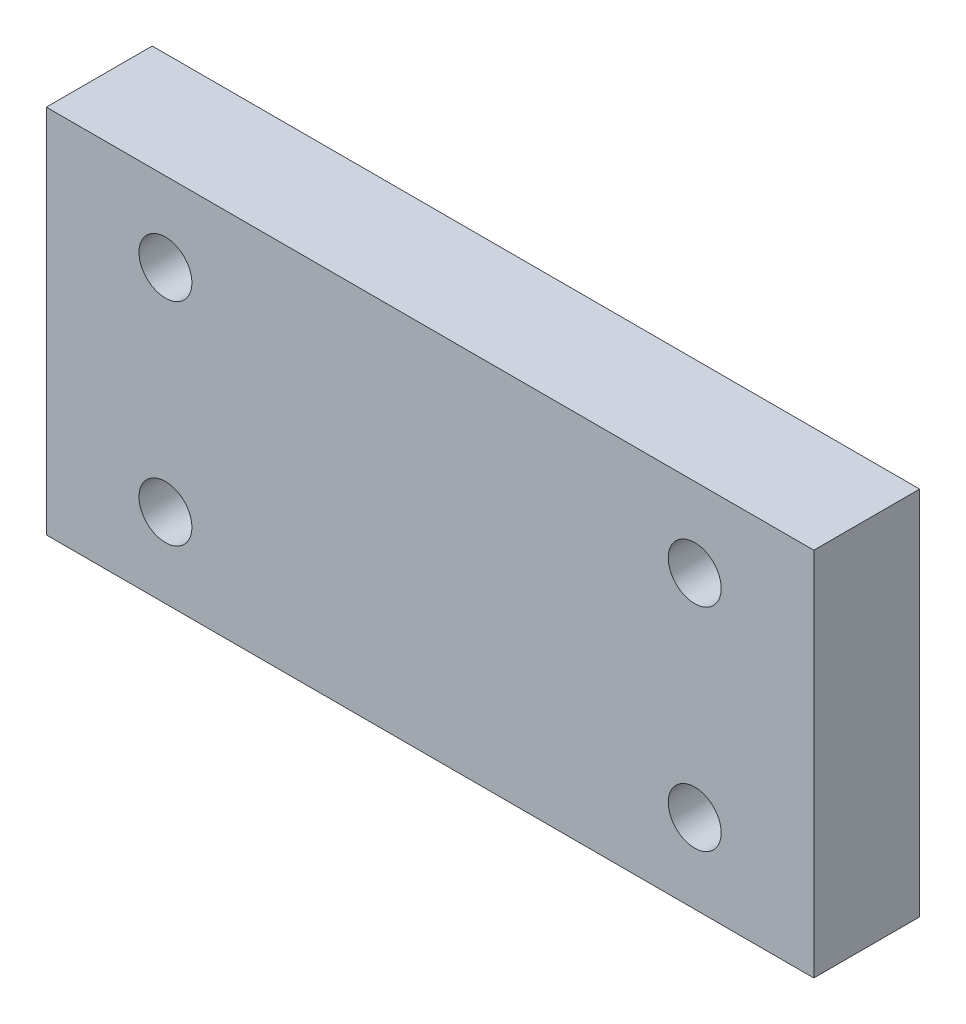
SolidWorks part; units mm, degrees
ref_plane "Front Plane" through (0, 0, 0) normal (0, 0, 1) x (1, 0, 0)
ref_plane "Top Plane" through (0, 0, 0) normal (0, 1, 0) x (1, 0, 0)
ref_plane "Right Plane" through (0, 0, 0) normal (1, 0, 0) x (0, 0, -1)
sketch "Sketch1" plane through (0, 0, 0) normal (0, 0, 1) x (1, 0, 0)
  line L0 (0, 137.9326) -> (0, -157.3569) construction
  line L1 (-145, -70) -> (145, -70)
  line L2 (-145, -70) -> (-145, 70)
  line L3 (-145, 70) -> (145, 70)
  line L4 (145, -70) -> (145, 70)
  line L5 (-145, -70) -> (145, 70) construction
  line L6 (-145, 70) -> (145, -70) construction
  circle A0 centre (-100, 40) radius 10
  circle A1 centre (-100, -40) radius 10
  circle A2 centre (100, -40) radius 10
  circle A3 centre (100, 40) radius 10
  point P0 (0, 0)
  dimension "D3" = 45
  dimension "D7" = 20
  dimension "D8" = 20
  dimension "D1" = 140
  dimension "D2" = 290
  dimension "D4" = 45
  dimension "D5" = 80
  dimension "D6" = 30
extrude "Boss-Extrude1" add sketch "Sketch1" along normal blind 40
